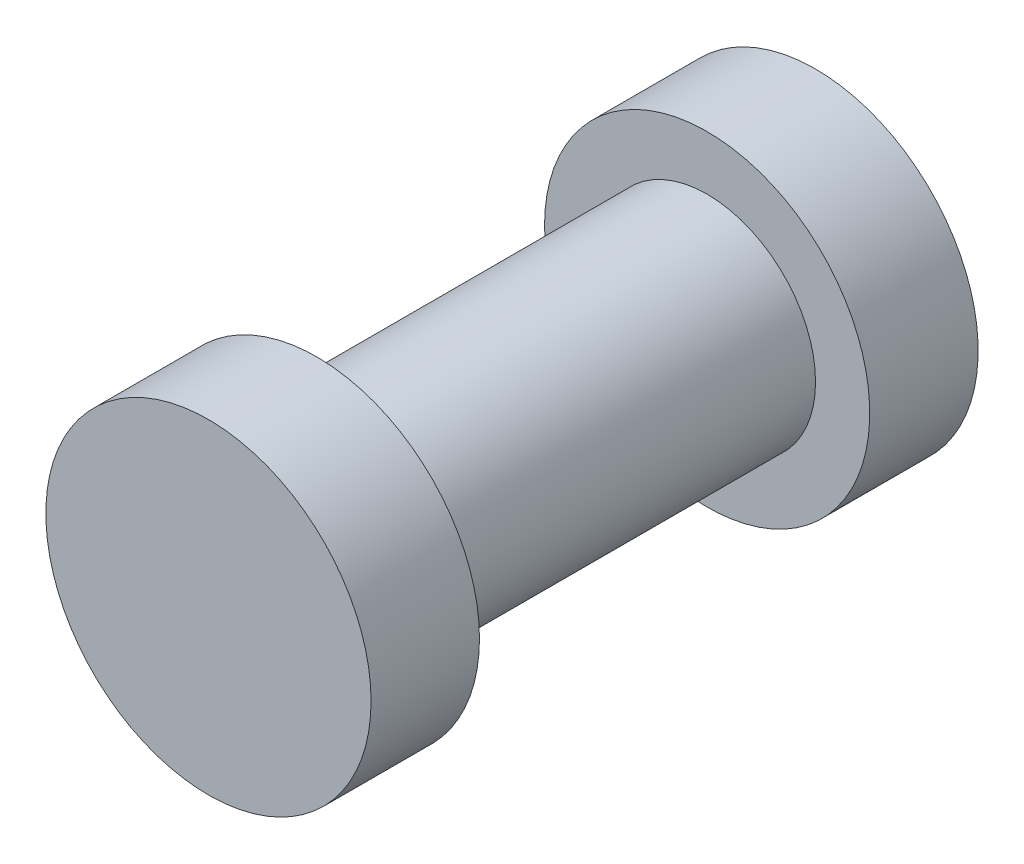
from build123d import *

# Parameters (mm, degrees)
SKETCH1_R           = 10
BOSS_EXTRUDE1_DEPTH = 36
SKETCH2_R           = 15
BOSS_EXTRUDE2_DEPTH = 10
BOSS_EXTRUDE3_START = 10
SKETCH3_R           = 15
BOSS_EXTRUDE3_DEPTH = 10


with BuildPart() as part:
    # Sketch1 → Boss-Extrude1 (new body)
    with BuildSketch(Plane.XY):
        Circle(SKETCH1_R)
    extrude(amount=BOSS_EXTRUDE1_DEPTH)

    # Sketch2 → Boss-Extrude2 (add)
    with BuildSketch(Plane.XY.offset(36)):
        Circle(SKETCH2_R)
    extrude(amount=BOSS_EXTRUDE2_DEPTH)

    # Sketch3 → Boss-Extrude3 (add)
    with BuildSketch(Plane(origin=(0, 0, 0), x_dir=(-1, 0, 0), z_dir=(0, 0, -1)).offset(BOSS_EXTRUDE3_START)):
        with Locations(Location((0, 0, 0), (0, 0, 180))):
            Circle(SKETCH3_R)
    extrude(amount=-BOSS_EXTRUDE3_DEPTH)


solid = part.part
